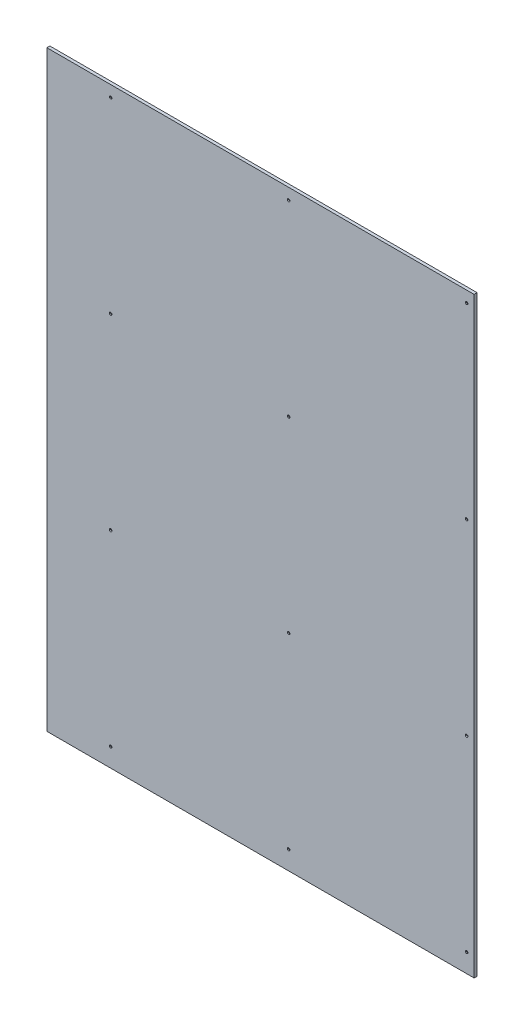
SolidWorks part; units mm, degrees
ref_plane "Front Plane" through (0, 0, 0) normal (0, 0, 1) x (1, 0, 0)
ref_plane "Top Plane" through (0, 0, 0) normal (0, 1, 0) x (1, 0, 0)
ref_plane "Right Plane" through (0, 0, 0) normal (1, 0, 0) x (0, 0, -1)
sketch "Sketch1" plane through (0, 0, 0) normal (0, 0, 1) x (1, 0, 0)
  line L1 (-570, 790) -> (570, 790)
  line L2 (-570, 790) -> (-570, -790)
  line L3 (-570, -790) -> (570, -790)
  line L4 (570, 790) -> (570, -790)
  line L5 (-570, 790) -> (570, -790) construction
  line L6 (-570, -790) -> (570, 790) construction
  point P0 (0, 0)
  dimension "D1" = 1140
  dimension "D2" = 1580
extrude "Boss-Extrude1" add sketch "Sketch1" along normal blind 8 contours L2 L1 L4 L3
sketch "Sketch2" plane through (0, 0, 8) normal (0, 0, 1) x (1, 0, 0)
  line L0 (-570, -790) -> (570, -790) construction
  line L1 (-570, 790) -> (-570, -790) construction
  circle A0 centre (-400, -240) radius 3.5
  circle A1 centre (75, -240) radius 3.5
  circle A2 centre (550, -240) radius 3.5
  circle A3 centre (-400, 260) radius 3.5
  circle A4 centre (75, 260) radius 3.5
  circle A5 centre (550, 260) radius 3.5
  circle A6 centre (-400, 760) radius 3.5
  circle A7 centre (75, 760) radius 3.5
  circle A8 centre (550, 760) radius 3.5
  circle A9 centre (-400, -740) radius 3.5
  circle A10 centre (75, -740) radius 3.5
  circle A11 centre (550, -740) radius 3.5
  dimension "D8" = 7
  dimension "D1" = 500
  dimension "D2" = 1000
  dimension "D3" = 1500
  dimension "D4" = 50
  dimension "D5" = 475
  dimension "D6" = 475
  dimension "D7" = 170
extrude "Cut-Extrude1" cut sketch "Sketch2" against normal blind 3
sketch "Sketch3" plane through (0, 0, 5) normal (0, 0, 1) x (1, 0, 0)
  circle A0 centre (550, -740) radius 3.5 construction
  circle A1 centre (75, -740) radius 3.5 construction
  circle A2 centre (-400, -740) radius 3.5 construction
  circle A3 centre (-400, -240) radius 3.5 construction
  circle A4 centre (75, -240) radius 3.5 construction
  circle A5 centre (550, -240) radius 3.5 construction
  circle A6 centre (550, 260) radius 3.5 construction
  circle A7 centre (75, 260) radius 3.5 construction
  circle A8 centre (-400, 260) radius 3.5 construction
  circle A9 centre (550, 760) radius 3.5 construction
  circle A10 centre (75, 760) radius 3.5 construction
  circle A11 centre (-400, 760) radius 3.5 construction
  circle A12 centre (550, -740) radius 3.5
  circle A13 centre (75, -740) radius 3.5
  circle A14 centre (-400, -740) radius 3.5
  circle A15 centre (-400, -240) radius 3.5
  circle A16 centre (75, -240) radius 3.5
  circle A17 centre (550, -240) radius 3.5
  circle A18 centre (550, 260) radius 3.5
  circle A19 centre (75, 260) radius 3.5
  circle A20 centre (-400, 260) radius 3.5
  circle A21 centre (550, 760) radius 3.5
  circle A22 centre (75, 760) radius 3.5
  circle A23 centre (-400, 760) radius 3.5
extrude "Cut-Extrude2" cut sketch "Sketch3" against normal blind 5 draft 45 draft outward yes
